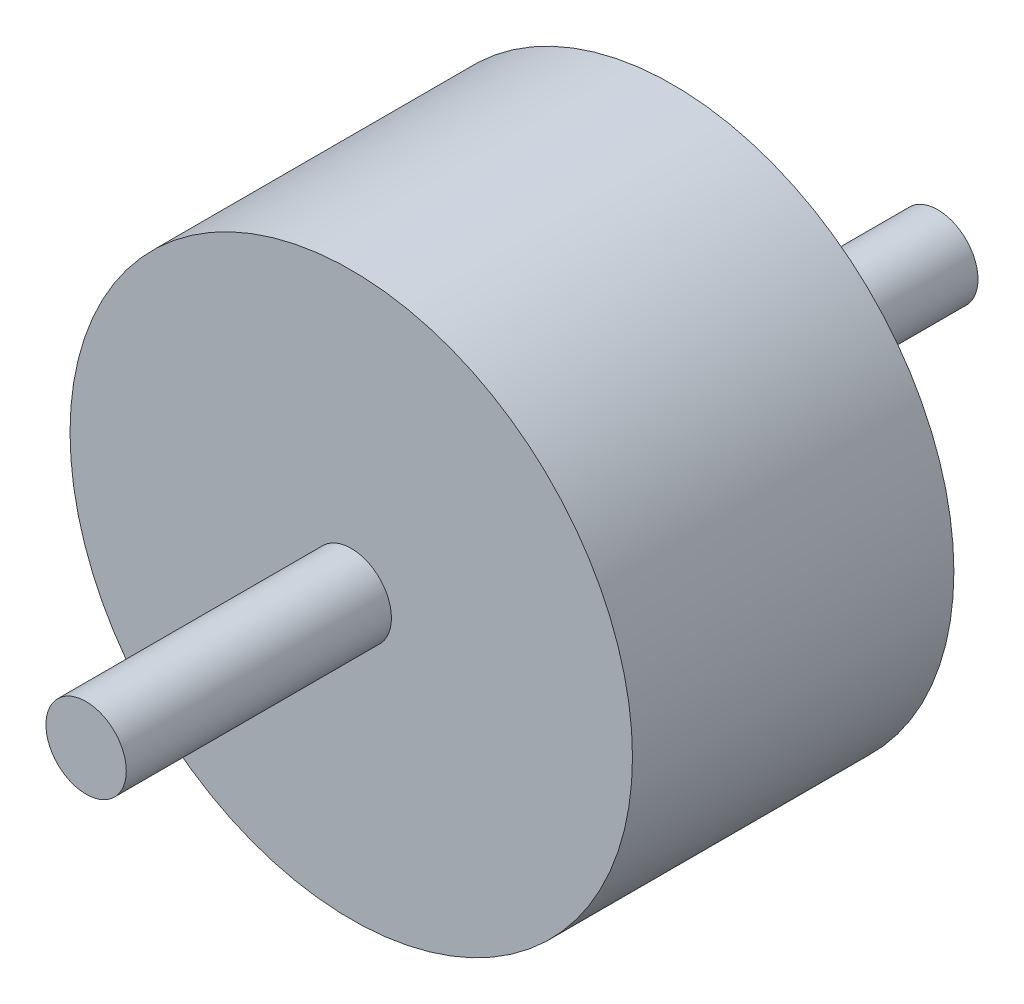
from build123d import *

# Parameters (mm, degrees)
SKETCH_1_R      = 35
EXTRUDE_1_DEPTH = 40
SKETCH_2_R      = 5
EXTRUDE_2_DEPTH = 33
EXTRUDE_START   = 33
SKETCH_3_R      = 5
EXTRUDE_3_DEPTH = 33


with BuildPart() as part:
    # 草图1 → 凸台-拉伸1 (new body)
    with BuildSketch(Plane.XY):
        Circle(SKETCH_1_R)
    extrude(amount=EXTRUDE_1_DEPTH)

    # 草图2 → 凸台-拉伸2 (add)
    with BuildSketch(Plane.XY.offset(40)):
        Circle(SKETCH_2_R)
    extrude(amount=EXTRUDE_2_DEPTH)

    # 草图3 → 凸台-拉伸3 (add)
    with BuildSketch(Plane(origin=(0, 0, 0), x_dir=(-1, 0, 0), z_dir=(0, 0, -1)).offset(EXTRUDE_START)):
        with Locations(Location((0, 0, 0), (0, 0, 180))):
            Circle(SKETCH_3_R)
    extrude(amount=-EXTRUDE_3_DEPTH)


solid = part.part
